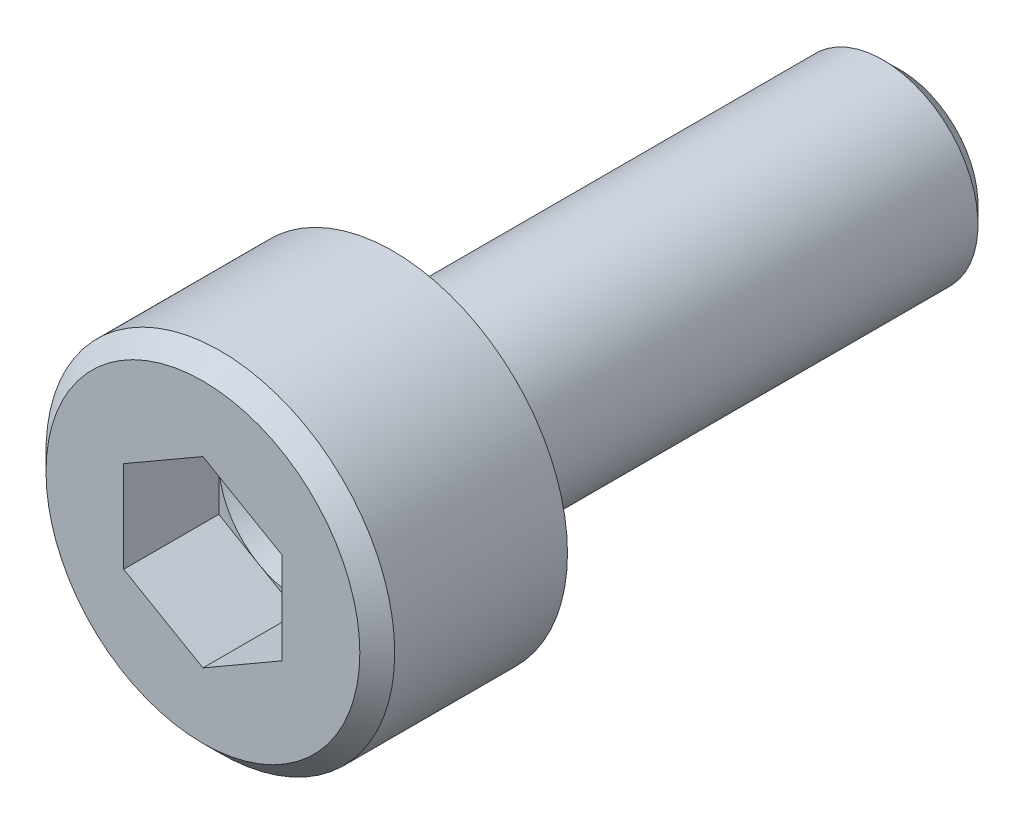
SolidWorks part; units mm, degrees
material "SUS304/0Cr18Ni9"
ref_plane "前视基准面" through (0, 0, 0) normal (0, 0, 1) x (1, 0, 0)
ref_plane "上视基准面" through (0, 0, 0) normal (0, 1, 0) x (1, 0, 0)
ref_plane "右视基准面" through (0, 0, 0) normal (1, 0, 0) x (0, 0, -1)
sketch "草图1" plane through (0, 0, 0) normal (0, 1, 0) x (1, 0, 0)
  line L0 (2.75, 0) -> (0, 0)
  line L1 (0, 0) -> (0, -3)
  line L2 (0, -3) -> (2.75, -3)
  line L3 (2.75, -3) -> (2.75, 0)
  line L4 (0, 0) -> (0, -3) construction
revolve "旋转1" add sketch "草图1" angle 360 about L4
sketch "草图2" plane through (0, 0, 0) normal (0, 0, -1) x (-1, 0, 0)
  circle A0 centre (0, 0) radius 1.5
extrude "凸台-拉伸1" add sketch "草图2" along normal blind 8
sketch "草图3" plane through (0, 0, 3) normal (0, 0, 1) x (1, 0, 0)
  line L0 (1.25, -0.7217) -> (1.25, 0.7217)
  line L1 (1.25, 0.7217) -> (0, 1.4434)
  line L2 (0, 1.4434) -> (-1.25, 0.7217)
  line L3 (-1.25, 0.7217) -> (-1.25, -0.7217)
  line L4 (-1.25, -0.7217) -> (0, -1.4434)
  line L5 (0, -1.4434) -> (1.25, -0.7217)
extrude "切除-拉伸1" cut sketch "草图3" against normal blind 1.5
ref_plane "基准面1" through (0, 0, 0) normal (0, -1, 0) x (1, 0, 0)
sketch "草图4" plane through (0, 0, 0) normal (0, -1, 0) x (1, 0, 0)
  line L0 (1.25, 1.5) -> (0, 1.5)
  line L1 (0, 1.5) -> (0, 0.7783)
  line L2 (0, 0.7783) -> (1.25, 1.5)
  line L3 (0, 1.5) -> (0, 0.7783) construction
revolve "切除-旋转1" cut sketch "草图4" angle 360 about L3
chamfer "倒角1" distance 0.275 angle 45 2 edges at (-1.5, 0, -8) (2.75, 0, 3)
